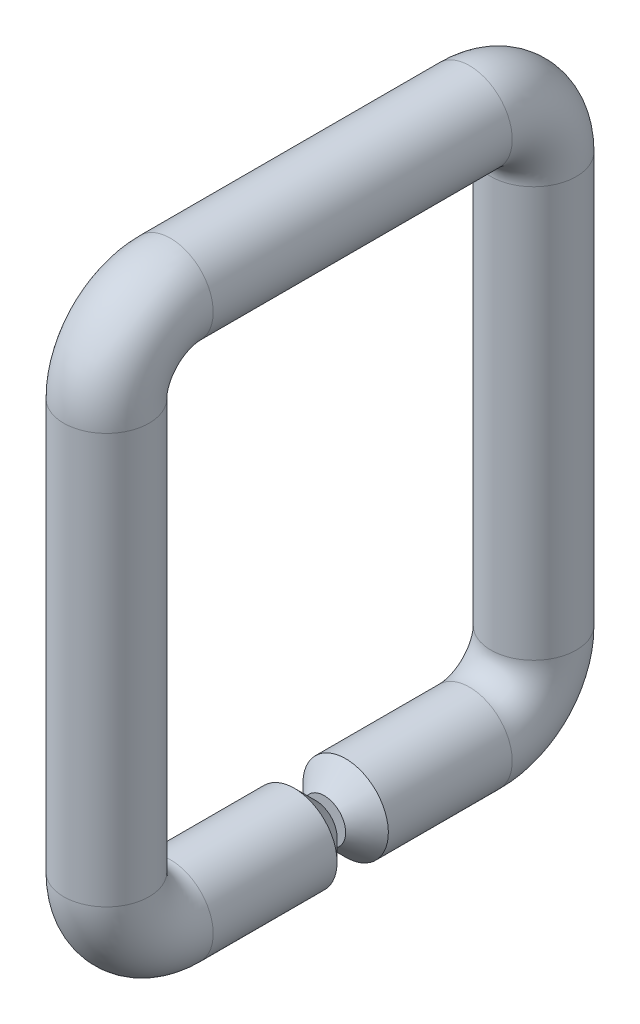
SolidWorks part; units mm, degrees
ref_plane "Front Plane" through (0, 0, 0) normal (0, 0, 1) x (1, 0, 0)
ref_plane "Top Plane" through (0, 0, 0) normal (0, 1, 0) x (1, 0, 0)
ref_plane "Right Plane" through (0, 0, 0) normal (1, 0, 0) x (0, 0, -1)
sketch "Sketch2" plane through (0, 0, 0) normal (0, 0, 1) x (1, 0, 0)
  circle A0 centre (0, 0) radius 10
  dimension "D1" = 20
sketch "Sketch4" plane through (0, 0, 0) normal (1, 0, 0) x (0, 0, -1)
  line L0 (0, 0) -> (-34, 0)
  line L1 (-49, 15) -> (-49, 111)
  line L2 (-34, 126) -> (36, 126)
  line L3 (51, 111) -> (51, 15)
  line L4 (36, 0) -> (2, 0)
  arc A0 (36, 126) -> (51, 111) centre (36, 111) cw
  arc A1 (-49, 111) -> (-34, 126) centre (-34, 111) cw
  arc A2 (51, 15) -> (36, 0) centre (36, 15) cw
  arc A3 (-49, 15) -> (-34, 0) centre (-34, 15) ccw
  point P9 (51, 126)
  point P12 (-49, 126)
  point P15 (51, 0)
  point P18 (-49, 0)
  dimension "D5" = 15
  dimension "D1" = 49
  dimension "D2" = 126
  dimension "D3" = 100
  dimension "D4" = 49
sweep "Sweep1" add profiles "Sketch2" path "Sketch4"
chamfer "Chamfer1" distance 5 angle 45 2 edges at (10, 0, -2) (10, 0, 0)
